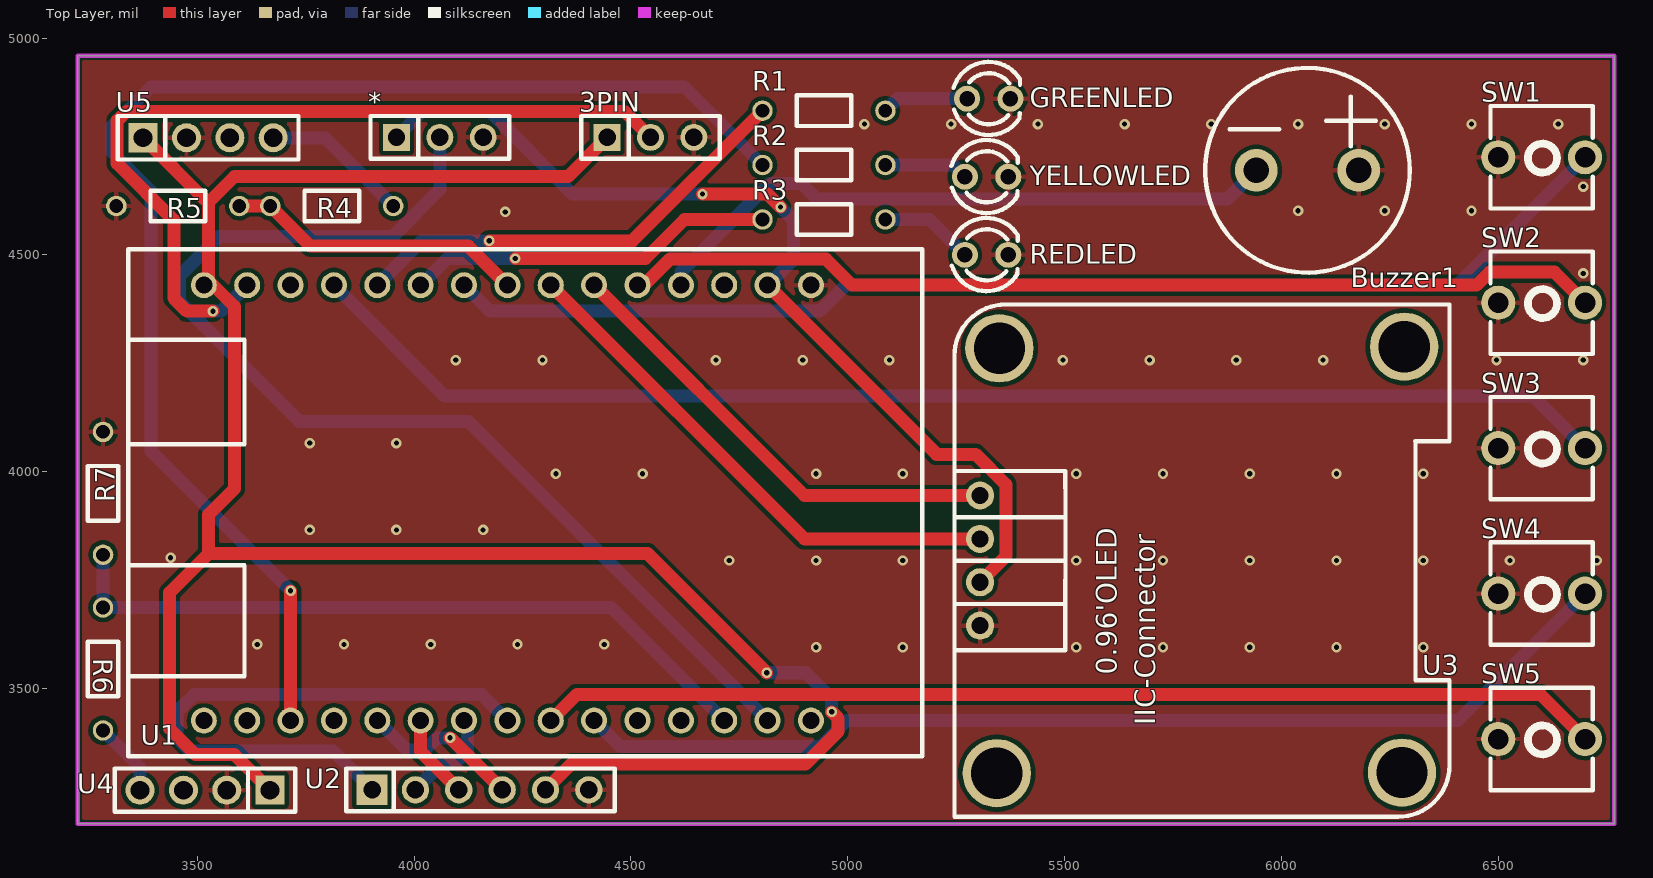
[diagram p0: Top Layer view]
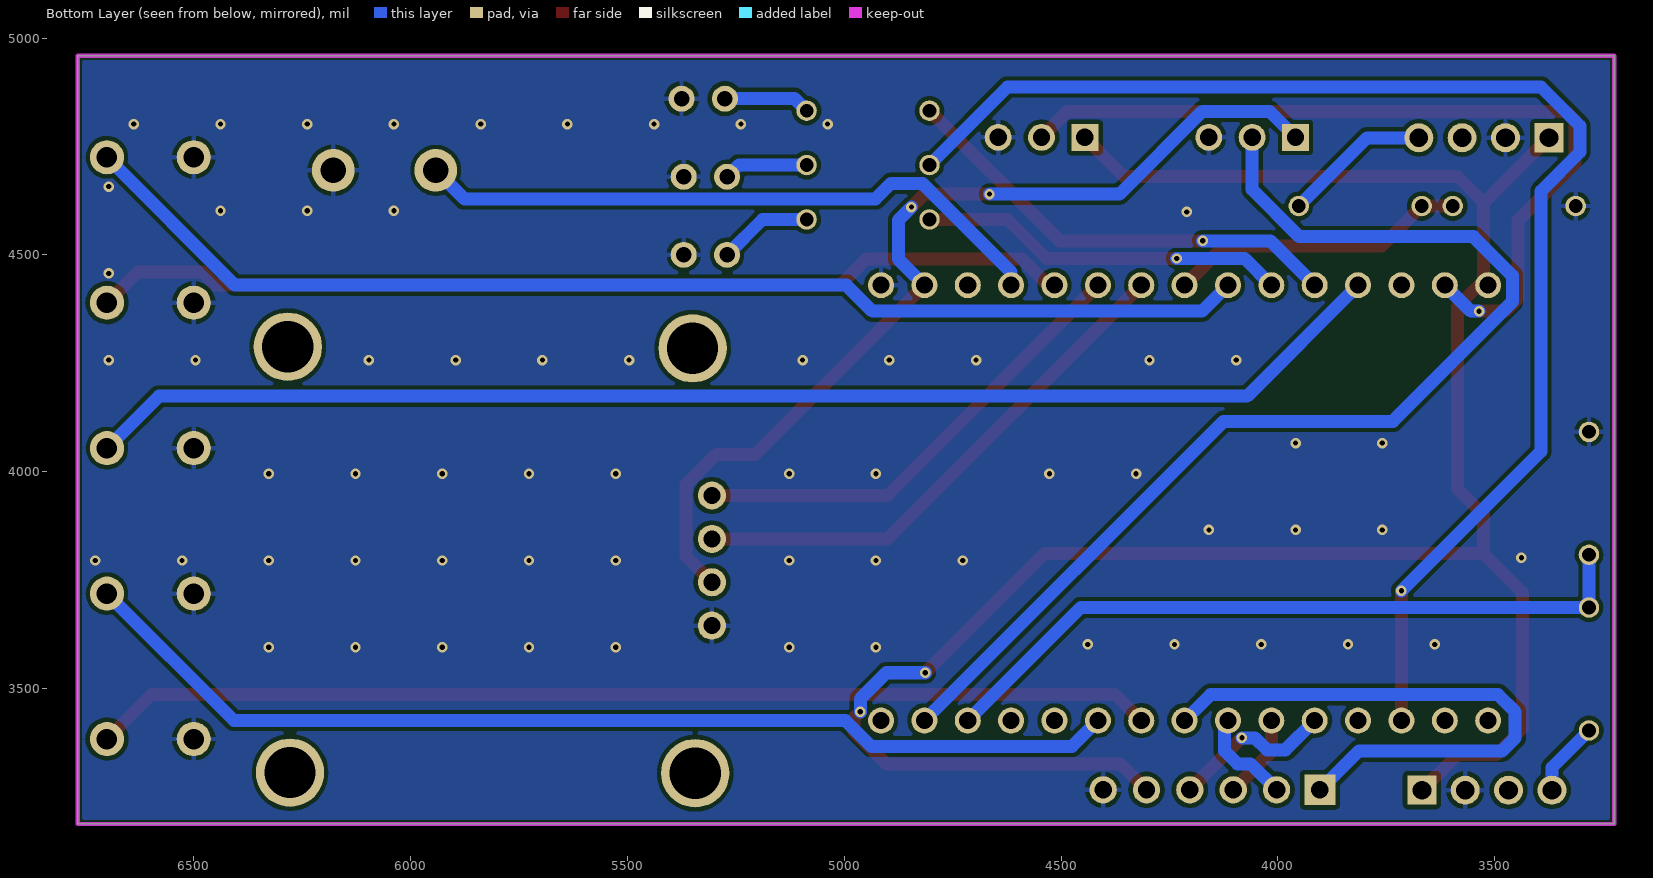
[diagram p1: Bottom Layer view, seen from below]
# Altium PCB MISC51777.pcbdoc
Units mil, origin at the board's own origin, x right, y up, seen from the top; angles counter-clockwise.
Board outline 3543.31 x 1771.65 mil, 2 copper layers (Top Layer, Bottom Layer), stack 62.206 mil thick; 23 components, 27 nets, 90 pads, 72 vias.

## Layer stack, top to bottom
Top Solder Mask Layer: solder mask 0.394, Dk 3.3
Top Layer: signal copper 1.379
Dielectric1: surface 59.449, FR4, Dk 4.5
Bottom Layer: signal copper 1.378
Bottom Solder Mask Layer: solder mask 0.394, Dk 3.3

## Board outline
3224.17,3187.52 6767.48,3187.52 6767.48,4959.17 3224.17,4959.17

## Design rules (kind name [scope] priority, off if disabled: settings)
BoardOutlineClearance copperThickness2oz_1 [All] p2 off: genericclearance=7.99 ignorepadtopadclearanceinfootprint=FALSE except(0: Arc-SplitContinuation Track-SplitContinuation SMDPad-SplitContinuation THPad-SplitContinuation Via-SplitContinuation Fill-SplitContinuation Region-SplitContinuation Poly-SplitContinuation Text-SplitContinuation Hole-SplitContinuation; 5.98: Arc-CutoutEdge Track-CutoutEdge SMDPad-CutoutEdge THPad-CutoutEdge Via-CutoutEdge Text-CutoutEdge; 6.89: Hole-OutlineEdge Hole-CutoutEdge; 10: Poly-OutlineEdge Poly-CutoutEdge; 11.81: Arc-OutlineEdge Track-OutlineEdge SMDPad-OutlineEdge THPad-OutlineEdge Via-OutlineEdge Fill-OutlineEdge Region-OutlineEdge Text-OutlineEdge Fill-CutoutEdge Region-CutoutEdge)
BoardOutlineClearance Plane_innerPlane_1 [All] p4 off: genericclearance=4.02 ignorepadtopadclearanceinfootprint=FALSE except(0: Arc-SplitContinuation Track-SplitContinuation SMDPad-SplitContinuation THPad-SplitContinuation Via-SplitContinuation Fill-SplitContinuation Region-SplitContinuation Poly-SplitContinuation Text-SplitContinuation Hole-SplitContinuation; 5.98: Arc-CutoutEdge Track-CutoutEdge SMDPad-CutoutEdge THPad-CutoutEdge Via-CutoutEdge Text-CutoutEdge; 6.89: Hole-OutlineEdge Hole-CutoutEdge; 10: Poly-OutlineEdge Poly-CutoutEdge; 11.81: Arc-OutlineEdge Track-OutlineEdge SMDPad-OutlineEdge THPad-OutlineEdge Via-OutlineEdge Fill-OutlineEdge Region-OutlineEdge Text-OutlineEdge Fill-CutoutEdge Region-CutoutEdge)
BoardOutlineClearance Copper_copperRegion_1 [All] p6 off: genericclearance=4.02 ignorepadtopadclearanceinfootprint=FALSE except(0: Arc-SplitContinuation Track-SplitContinuation SMDPad-SplitContinuation THPad-SplitContinuation Via-SplitContinuation Fill-SplitContinuation Region-SplitContinuation Poly-SplitContinuation Text-SplitContinuation Hole-SplitContinuation; 5.98: Arc-CutoutEdge Track-CutoutEdge SMDPad-CutoutEdge THPad-CutoutEdge Via-CutoutEdge Text-CutoutEdge; 6.89: Hole-OutlineEdge Hole-CutoutEdge; 10: Poly-OutlineEdge Poly-CutoutEdge; 11.81: Arc-OutlineEdge Track-OutlineEdge SMDPad-OutlineEdge THPad-OutlineEdge Via-OutlineEdge Fill-OutlineEdge Region-OutlineEdge Text-OutlineEdge Fill-CutoutEdge Region-CutoutEdge)
BoardOutlineClearance copperThickness1oz_1 [All] p8: genericclearance=4.02 ignorepadtopadclearanceinfootprint=FALSE except(0: Arc-SplitContinuation Track-SplitContinuation SMDPad-SplitContinuation THPad-SplitContinuation Via-SplitContinuation Fill-SplitContinuation Region-SplitContinuation Poly-SplitContinuation Text-SplitContinuation Hole-SplitContinuation; 5.98: Arc-CutoutEdge Track-CutoutEdge SMDPad-CutoutEdge THPad-CutoutEdge Via-CutoutEdge Text-CutoutEdge; 6.89: Hole-OutlineEdge Hole-CutoutEdge; 10: Poly-OutlineEdge Poly-CutoutEdge; 11.81: Arc-OutlineEdge Track-OutlineEdge SMDPad-OutlineEdge THPad-OutlineEdge Via-OutlineEdge Fill-OutlineEdge Region-OutlineEdge Text-OutlineEdge Fill-CutoutEdge Region-CutoutEdge)
Clearance copperThickness2oz [All] p1 off: gap=7.99 ignorepadtopadclearanceinfootprint=FALSE except(5.98: SMDPad-Track SMDPad-SMDPad THPad-Track SMDPad-THPad THPad-THPad Track-Via SMDPad-Via THPad-Via Via-Via Fill-SMDPad Region-SMDPad Fill-THPad Region-THPad Fill-Via Region-Via Fill-Fill Fill-Region Region-Region Arc-Track Arc-SMDPad Arc-THPad Arc-Via Fill-Arc Region-Arc Arc-Arc Text-Track SMDPad-Text Text-THPad Text-Via Fill-Text Region-Text Arc-Text Text-Text; 6.89: Hole-Track Hole-SMDPad Hole-THPad Hole-Via Fill-Hole Region-Hole Hole-Arc Hole-Text; 10: Poly-Track Poly-SMDPad Poly-THPad Poly-Via Poly-Fill Poly-Region Poly-Poly Poly-Arc Poly-Text Poly-Hole; 11.81: Fill-Track Region-Track)
Clearance Plane_innerPlane [All] p3 off: gap=4.02 ignorepadtopadclearanceinfootprint=FALSE except(5.98: SMDPad-Track SMDPad-SMDPad THPad-Track SMDPad-THPad THPad-THPad Track-Via SMDPad-Via THPad-Via Via-Via Fill-SMDPad Region-SMDPad Fill-THPad Region-THPad Fill-Via Region-Via Fill-Fill Fill-Region Region-Region Arc-Track Arc-SMDPad Arc-THPad Arc-Via Fill-Arc Region-Arc Arc-Arc Text-Track SMDPad-Text Text-THPad Text-Via Fill-Text Region-Text Arc-Text Text-Text; 6.89: Hole-Track Hole-SMDPad Hole-THPad Hole-Via Fill-Hole Region-Hole Hole-Arc Hole-Text; 10: Poly-Track Poly-SMDPad Poly-THPad Poly-Via Poly-Fill Poly-Region Poly-Poly Poly-Arc Poly-Text Poly-Hole; 11.81: Fill-Track Region-Track)
Clearance Copper_copperRegion [All] p5 off: gap=4.02 ignorepadtopadclearanceinfootprint=FALSE except(5.98: SMDPad-Track SMDPad-SMDPad THPad-Track SMDPad-THPad THPad-THPad Track-Via SMDPad-Via THPad-Via Via-Via Fill-SMDPad Region-SMDPad Fill-THPad Region-THPad Fill-Via Region-Via Fill-Fill Fill-Region Region-Region Arc-Track Arc-SMDPad Arc-THPad Arc-Via Fill-Arc Region-Arc Arc-Arc Text-Track SMDPad-Text Text-THPad Text-Via Fill-Text Region-Text Arc-Text Text-Text; 6.89: Hole-Track Hole-SMDPad Hole-THPad Hole-Via Fill-Hole Region-Hole Hole-Arc Hole-Text; 10: Poly-Track Poly-SMDPad Poly-THPad Poly-Via Poly-Fill Poly-Region Poly-Poly Poly-Arc Poly-Text Poly-Hole; 11.81: Fill-Track Region-Track)
Clearance copperThickness1oz [All] p7: gap=4.02 ignorepadtopadclearanceinfootprint=FALSE except(5.98: SMDPad-Track SMDPad-SMDPad THPad-Track SMDPad-THPad THPad-THPad Track-Via SMDPad-Via THPad-Via Via-Via Fill-SMDPad Region-SMDPad Fill-THPad Region-THPad Fill-Via Region-Via Fill-Fill Fill-Region Region-Region Arc-Track Arc-SMDPad Arc-THPad Arc-Via Fill-Arc Region-Arc Arc-Arc Text-Track SMDPad-Text Text-THPad Text-Via Fill-Text Region-Text Arc-Text Text-Text; 6.89: Hole-Track Hole-SMDPad Hole-THPad Hole-Via Fill-Hole Region-Hole Hole-Arc Hole-Text; 10: Poly-Track Poly-SMDPad Poly-THPad Poly-Via Poly-Fill Poly-Region Poly-Poly Poly-Arc Poly-Text Poly-Hole; 11.81: Fill-Track Region-Track)
DiffPairsRouting differentialPair [All] p1: maxlimit=6 minlimit=6 mostfreqgap=6 toplayer_minwidth=5 toplayer_prefwidth=10 toplayer_maxwidth=100 toplayer_mingap=6 toplayer_prefgap=6 toplayer_maxgap=6 bottomlayer_minwidth=5 bottomlayer_prefwidth=10 bottomlayer_maxwidth=100 bottomlayer_mingap=6 bottomlayer_prefgap=6 bottomlayer_maxgap=6 maxuncoupledlength=10
HoleToHoleClearance otherClearance [All] p1: gap=11.81 allowstackedmicrovias=TRUE
Length netLength [All] p1: minlimit=0 maxlimit=0
PasteMaskExpansion pasteMaskExpansion [All] p1: expansion=0
PlaneConnect innerPlane [All] p1: planeconnectstyle=Relief reliefexpansion=20 reliefentries=4 reliefconductorwidth=10 reliefairgap=10
PolygonConnect copperRegion [All] p1: connectstyle=Relief reliefconductorwidth=10 reliefentries=4 polygonreliefangle="90 Angle" airgapwidth=10 via.connectstyle=Relief via.reliefconductorwidth=10 via.reliefentries=4 via.polygonreliefangle="90 Angle" via.airgapwidth=10
RoutingVias viaSize [All] p1: holewidth=12.01 width=24.02 viastyle="Through Hole" minholewidth=11.81 minwidth=19.68 maxholewidth=248.03 maxwidth=393.7
SolderMaskExpansion solderMaskExpansion [IsVia] p1: expansion=-1000 istentingtop=TRUE
SolderMaskExpansion solderMaskExpansion [All] p2: expansion=2.01 istentingtop=FALSE
Width copperThickness2oz_2 [All] p1 off: maxlimit=100 minlimit=8 preferedwidth=10
Width copperThickness1oz_2 [All] p2: maxlimit=100 minlimit=5 preferedwidth=30

## Components (designator, comment, footprint, x,y, rotation, side; value= is the part's Value field where it differs from the comment)
3PIN "" HDR-TH_3P-P2.54-V-F 4545,4770.79 r0 top
* "DHT11" HDR-TH_3P-P2.54-V-F 4059.21,4770.79 r0 top
Buzzer1 "Buzzer" BUZ-TH_BD12.0-P6.00-D0.9-RD 6060,4695 r0 top
GREENLED "LED_3M" LED_TH-3mm 5325,4860 r0 top
R1 "220" Res_1/8W 4945,4830 r0 top
R2 "220" Res_1/8W 4945,4704.56 r0 top
R3 "220" Res_1/8W 4945,4579.13 r0 top
R4 "15kΩ" Res_1/8W 3810,4615 r180 top
R5 "27kΩ" Res_1/8W 3455,4615 r180 top
R6 "15kΩ" Res_1/8W 3280,3545 r270 top
R7 "27kΩ" Res_1/8W 3285,3950 r90 top
REDLED "LED_3M" LED_TH-3mm 5320,4500 r0 top
SW1 "SELECT" KEY-TH_2P-L6.0-W6.0-P5.00 6600,4725 r0 top
SW2 "CONFIRM" KEY-TH_2P-L6.0-W6.0-P5.00 6600,4389.6 r0 top
SW3 "INCREASE" KEY-TH_2P-L6.0-W6.0-P5.00 6600,4054.21 r0 top
SW4 "DECREASE" KEY-TH_2P-L6.0-W6.0-P5.00 6600,3718.81 r0 top
SW5 "Off" KEY-TH_2P-L6.0-W6.0-P5.00 6600,3383.41 r0 top
U1 "ESP32-C6" HDR-TH_33P-P2.54-V-R2-C15-S2.54_C9041 4215,4430 r180 top
U2 "MicroSD" HDR-TH_6P-P2.54-V-F 4152.89,3266.29 r0 top
U3 "OLED_SSD1306" 0.96OLED_4P 5305,3795 r90 top
U4 "MQ7" HDR-TH_4P-P2.54-V-F 3517.89,3265.51 r180 top
U5 "MQ135" HDR-TH_4P-P2.54-V-F 3525,4770 r0 top
YELLOWLED "LED_3M" LED_TH-3mm 5320,4680 r0 top

## Footprints (in the part's own frame and the unit in brackets; to place one, negate y for a bottom-side part, rotate by r counter-clockwise, add the part's x,y. Pads: shape width x height; smd on the part's side, far side on the other; paste and mask are expansions set on the pad)
0.96OLED_4P [mm]
  round 1.65 hole 1 copper offset 0,0: 1(-3.81,-0.001) 2(-1.27,0.002) 3(1.27,0.002) 4(3.81,0.002)
  round 4 hole 3: 5(-12.455,-0.98) 5(-12.42,-24.71) 5(12.435,-1.13) 5(12.525,-24.84)
  silkscreen extent -15,-27.5 15,1.5
BUZ-TH_BD12.0-P6.00-D0.9-RD [mm]
  round 2.5 hole 1.5 paste+0 mask+0.05: 1(-3,0) 2(3,0)
  silkscreen extent -5.99,-5.99 5.99,5.99
HDR-TH_3P-P2.54-V-F [mil]
  rect 62x62 hole 40.16: 1(-100,0)
  round 62 hole 40.16: 2(0,0) 3(100,0)
  silkscreen extent -160,-49 160,49
HDR-TH_4P-P2.54-V-F [mm]
  rect 1.7x1.7 hole 1.1: 1(-3.81,0)
  round 1.7 hole 1.1: 2(-1.27,0) 3(1.27,0) 4(3.81,0)
  silkscreen extent -5.29,-1.27 5.29,1.27
HDR-TH_6P-P2.54-V-F [mm]
  rect 1.8x1.8 hole 1.02: 1(-6.35,0)
  round 1.6 hole 1.02: 2(-3.81,0) 3(-1.27,0) 4(1.27,0) 5(3.81,0) 6(6.35,0)
  silkscreen extent -7.87,-1.25 7.87,1.25
HDR-TH_33P-P2.54-V-R2-C15-S2.54_C9041 [mil]
  round 60 hole 39.37: 1(-700,0) 2(-600,0) 3(-500,0) 4(-400,0) 5(-300,0) 6(-200,0) 7(-100,0) 8(0,0) 9(100,0) 10(200,0) 11(300,0) 12(400,0) 13(500,0) 14(600,0) 15(700,0) 16(-700,1003.94) 17(-600,1003.94) 18(-500,1003.94) 19(-400,1003.94) 20(-300,1003.94) 21(-200,1003.94) 22(-100,1003.94) 23(0,1003.94) 24(100,1003.94) 25(200,1003.94) 26(300,1003.94) 27(400,1003.94) 28(500,1003.94) 29(600,1003.94) 30(700,1003.94)
  silkscreen extent -957,-83 874,1087
KEY-TH_2P-L6.0-W6.0-P5.00 [mm]
  round 2 hole 1.2: 1(-2.54,0) 2(2.54,0)
  silkscreen extent -3,-3 3,3
LED_TH-3mm [mil]
  round 60 hole 36 paste+0 mask+2: 1(-50,0) 2(50,0)
  silkscreen extent -81,-84 72,85
Res_1/8W [mil]
  round 47.2 hole 31.5 paste+0 mask+2: 1(-141.7,2.48) 2(141.7,2.48)
  silkscreen extent -63,-33 63,38

## Via types
v1: diameter 24.02, hole 12, Top Layer to Bottom Layer, 72 vias

## Nets (pads, with @x,y where several pads share a name; then routed paths per layer and width w, separated by ;. In a path a pad name is that pad's centre, name@x,y a point inside that pad or via, vN(x,y) a via of type N, cw(c..) or ccw(c..) an arc to the next point about the centre after c; other vN are vias at no path point)
3V3: *.1 U1.2 U3.2 | length 2209.7
  Top Layer w30: v1(4665,4640) 4815,4640 v1(4845,4610) ; U1.2 5205,4040 5295,4040 5364.95,3970.05 5364.95,3805 U3.2@5304.95,3745
  Bottom Layer w30: *.1 4019.21,4830.79 4174.21,4830.79 4365,4640 v1(4665,4640) ; U1.2 4875,4490 4875,4580 v1(4845,4610)
5V: 3PIN.1 U1.15 U2.5 U4.1 U5.1 | length 5188.1
  Top Layer w30: U5.1 3524.21,4620.79 3525.79,4620.79 ; U1.15 U1.15@3525.79,4440.79 ; U4.1 3585.79,3347.6 3495.79,3347.6 3435.79,3407.6 3435.79,3720.79 3525.79,3810.79 ; U2.5 4362.89,3326.29 4902.89,3326.29 4977.89,3401.29 4977.89,3431.29 v1(4962.89,3446.29) ; 3PIN.1 4355,4680.79 3585.79,4680.79 3525.79,4620.79 ; v1(4812.89,3536.29) 4538.39,3810.79 3525.79,3810.79 ; 3525.79,3810.79 3525.79,3900.79 3585.79,3960.79 3585.79,4380.79 U1.15@3525.79,4440.79 ; U1.15@3525.79,4440.79 3525.79,4620.79
  Bottom Layer w30: v1(4812.89,3536.29) 4902.89,3536.29 4962.89,3476.29 v1(4962.89,3446.29)
$1N5: Buzzer1.1 U1.4 | length 1484
  Bottom Layer w30: U1.4 4615,4460 4820,4665 4891.89,4665 4927.87,4629.02 5875.91,4629.02 Buzzer1.1
$1N6: GREENLED.1 R1.2 | length 199.7
  Bottom Layer w30: R1.2 5114.22,4860 GREENLED.1
$1N7: R3.2 REDLED.1 | length 217.1
  Bottom Layer w30: R3.2 5188.39,4581.61 REDLED.1
$1N10: SW1.2 U1.9 | length 2756.9
  Bottom Layer w30: U1.9 4175,4370 4935,4370 4995,4430 6405,4430 SW1.2
$1N11: SW2.2 U1.5 | length 2276.3
  Top Layer w30: U1.5 4529.6,4430 4589.6,4490 4949.6,4490 5009.6,4430 6449.6,4430 6479.6,4460 6629.6,4460 SW2.2
$1N12: SW3.2 U1.12 | length 3040.7
  Bottom Layer w30: U1.12 4070.79,4174.21 6580,4174.21 SW3.2
$1N13: SW4.2 U1.21 | length 2456
  Bottom Layer w30: U1.21 4475,3366.06 4937.26,3366.06 4997.26,3426.06 6407.26,3426.06 SW4.2
$1N14: SW5.2 U1.22 | length 2452.4
  Top Layer w30: U1.22 4375,3486.06 6597.35,3486.06 SW5.2
$1N15: R1.1 U1.11 | length 1055
  Top Layer w30: v1(4173.3,4532.48) 4503.3,4532.48 R1.1
  Bottom Layer w30: U1.11 4017.48,4532.48 v1(4173.3,4532.48)
$1N16: R2.1 U1.28 | length 3153.3
  Top Layer w30: U1.28 v1(3715,3725.34)
  Bottom Layer w30: v1(3715,3725.34) 3393.3,4047.04 3393.3,4647.04 3303.3,4737.04 3303.3,4797.04 3393.3,4887.04 4623.3,4887.04 R2.1
$1N17: R3.1 U1.10 | length 851.1
  Top Layer w30: v1(4233.3,4491.61) 4533.3,4491.61 4623.3,4581.61 R3.1
  Bottom Layer w30: U1.10 4076.61,4491.61 v1(4233.3,4491.61)
$1N18: R2.2 YELLOWLED.1 | length 194.5
  Bottom Layer w30: R2.2 5242.96,4707.04 YELLOWLED.1
$1N26: U1.6 U3.4 | length 1090.8
  Top Layer w30: U1.6 4900,3945 U3.4@5304.95,3945
$1N27: U1.7 U3.3 | length 1232.3
  Top Layer w30: U1.7 4900,3845 U3.3@5304.95,3845
$1N28: U1.23 U2.1 | length 1363.1
  Bottom Layer w30: U2.1 3812.89,3356.29 3482.89,3356.29 3452.89,3386.29 3452.89,3446.29 3492.66,3486.06 4155,3486.06 U1.23
$1N29: U1.24 U2.2 | length 230.3
  Bottom Layer w30: U2.2 4062.89,3326.29 4092.89,3326.29 4122.89,3356.29 4122.89,3418.18 U1.24
$1N30: U1.25 U2.3 | length 196.2
  Top Layer w30: U1.25 4015,3354.18 U2.3
$1N31: U1.26 U2.4 | length 377.1
  Top Layer w30: v1(4082.89,3386.29) U2.4
  Bottom Layer w30: U1.26 3982.61,3358.45 4025.04,3358.45 4052.89,3386.29 v1(4082.89,3386.29)
$1N36: *.2 U1.17 | length 2618.2
  Bottom Layer w30: *.2 4059.21,4650.79 3950.28,4541.85 3549.21,4541.85 3459.21,4451.85 3459.21,4391.85 3735,4116.06 4125,4116.06 U1.17
$1N38: 3PIN.2 U1.14 | length 1933.7
  Top Layer w30: v1(3535.79,4370) 3475.79,4370 3445.79,4400 3445.79,4580 3315,4710.79 3315,4809.25 3336.54,4830.79 4485,4830.79 3PIN.2
  Bottom Layer w30: v1(3535.79,4370) 3555,4370 U1.14
$1N3471: R4.1 U5.4 | length 341.9
  Bottom Layer w30: U5.4 3794.22,4770 R4.1
$1N3474: R4.2 R5.1 U1.8 | length 693.9
  Top Layer w30: R5.1 R4.2 3760.82,4520 4125,4520 U1.8
$1N3564: R6.2 U4.4 | length 173.2
  Bottom Layer w30: R6.2 3367.89,3317.89 U4.4
$1N3567: R6.1 R7.1 U1.18 | length 1662.1
  Bottom Layer w30: R7.1 R6.1 4454.36,3686.7 U1.18
GND: 3PIN.3 *.3 Buzzer1.2 GREENLED.2 R5.2 R7.2 REDLED.2 SW1.1 SW2.1 SW3.1 SW4.1 SW5.1 U1.1 U2.6 U3.1 U4.2 U5.2 YELLOWLED.2
  other v1: 4926.83,3595.16 5126.83,3595.16 5526.83,3595.16 5726.83,3595.16 5926.83,3595.16 6126.83,3595.16 6326.83,3595.16 3638.27,3601.62 3838.27,3601.62 4038.27,3601.62 4238.27,3601.62 4438.27,3601.62 4726.83,3795.16 4926.83,3795.16 5126.83,3795.16 5526.83,3795.16 5726.83,3795.16 5926.83,3795.16 6126.83,3795.16 6326.83,3795.16 6526.83,3795.16 6726.83,3795.16 3438.27,3801.62 3759.06,3865.81 3959.06,3865.81 4159.06,3865.81 4326.83,3995.16 4526.83,3995.16 4926.83,3995.16 5126.83,3995.16 5526.83,3995.16 5726.83,3995.16 5926.83,3995.16 6126.83,3995.16 6326.83,3995.16 3759.06,4065.81 3959.06,4065.81 4095.91,4257.3 4295.91,4257.3 4695.91,4257.3 4895.91,4257.3 5095.91,4257.3 5495.91,4257.3 5695.91,4257.3 5895.91,4257.3 6095.91,4257.3 6495.91,4257.3 6695.91,4257.3 6695.91,4457.3 4210.24,4599.1 6038.27,4601.62 6238.27,4601.62 6438.27,4601.62 6695.91,4657.3 5038.27,4801.62 5238.27,4801.62 5438.27,4801.62 5638.27,4801.62 5838.27,4801.62 6038.27,4801.62 6238.27,4801.62 6438.27,4801.62 6638.27,4801.62
pads on no net: U1.3 U1.13 U1.16 U1.19 U1.20 U1.27 U1.29 U1.30 U3.5 U4.3 U5.3

## Polygon pours and split planes (outlines as drawn)
GND on Top Layer (solid, remove dead copper, pour order 0): 3000,5140 3000,3025 6925,3025 6925,5140
GND on Bottom Layer (solid, remove dead copper, pour order 2): 3095,5085 3095,3000 6965,3000 6965,5085

## Keep-outs
Board Outline Layer:
  the board outline again, w10